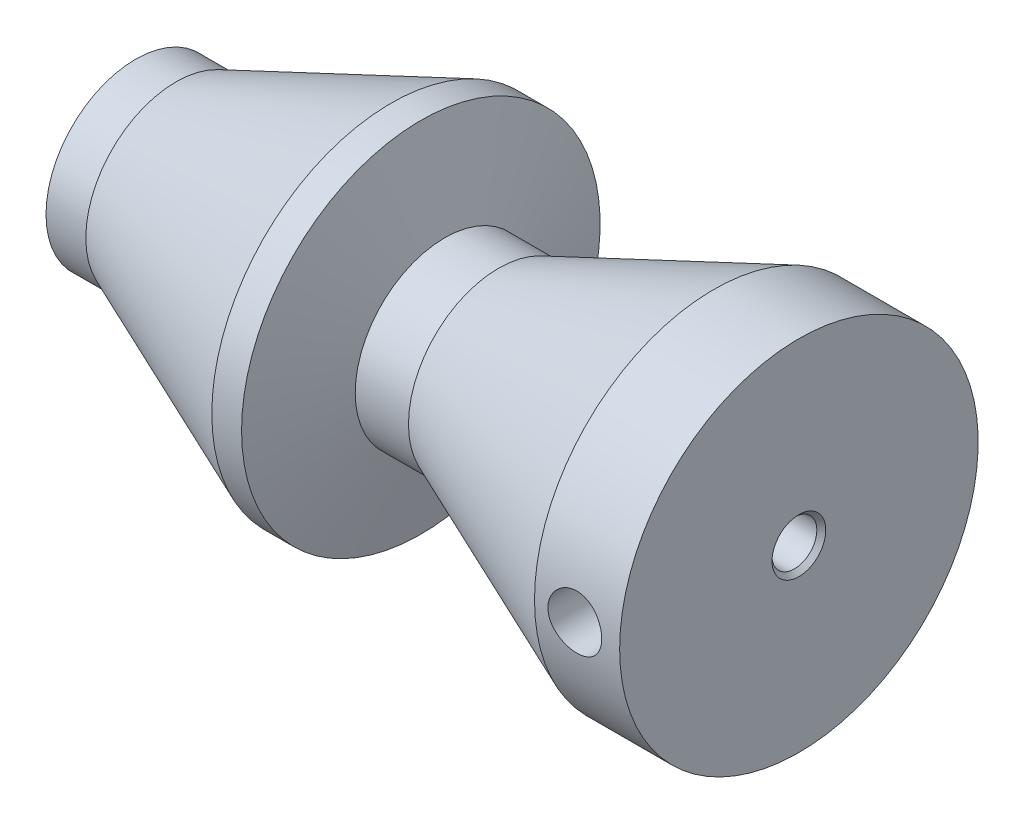
SolidWorks part; units mm, degrees
ref_plane "前视基准面" through (0, 0, 0) normal (0, 0, 1) x (1, 0, 0)
ref_plane "上视基准面" through (0, 0, 0) normal (0, 1, 0) x (1, 0, 0)
ref_plane "右视基准面" through (0, 0, 0) normal (1, 0, 0) x (0, 0, -1)
sketch "草图1" plane through (0, 0, 0) normal (0, 0, 1) x (1, 0, 0)
  line L0 (0, 0) -> (236.8731, 0) construction
  line L1 (4.5, 10) -> (0, 10)
  line L2 (4.5, 10.0589) -> (28.5, 20)
  line L3 (28.5, 20) -> (31.8205, 20)
  line L4 (31.8205, 20) -> (34.5, 10)
  line L5 (34.5, 10) -> (40.5, 10)
  line L6 (40.5, 10.0589) -> (64.5, 20)
  line L7 (64.5, 20) -> (74, 20)
  line L8 (74, 20) -> (74, 0)
  line L9 (40.5, 10.0589) -> (40.5, 10)
  line L10 (0, 10) -> (0, 0)
  line L11 (4.5, 10.0589) -> (4.5, 10)
  line L12 (0, 0) -> (74, 0)
  dimension "D1" = 4.5
  dimension "D2" = 22.5
  dimension "D3" = 74
  dimension "D4" = 9.5
  dimension "D5" = 20
  dimension "D6" = 36
  dimension "D7" = 22.5
  dimension "D8" = 10
  dimension "D9" = 36
  dimension "D10" = 6
  dimension "D11" = 105
revolve "旋转1" add sketch "草图1" angle 360 about L0
hole_wizard "M6 螺纹孔1" positions "草图3" profile "草图2" tap size "M6" standard "GB"
sketch "草图3" plane through (74, 0, 0) normal (1, 0, 0) x (0, 0, -1)
  point P0 (0, 0)
sketch "草图2" plane through (74, 0, 0) normal (0, 1, 0) x (0, 0, -1)
  line L0 (0, 0) -> (0, 18.5022)
  line L1 (0, 18.5022) -> (2.5, 17)
  line L2 (2.5, 17) -> (2.5, 0)
  line L5 (2.5, 0) -> (0, 0)
  line L10 (0, 18.5022) -> (-2.5, 17) construction
  line L11 (0, -6.35) -> (0, 107.95) construction
  dimension "螺纹孔钻头直径" = 5
  dimension "螺纹孔钻头深度" = 17
  dimension "导头角度" = 118
cosmetic thread "孔螺蚊线1" parameters "D1"=12, "D2"=6
chamfer "倒角1" distance 0.5 angle 45 1 edges at (74, 0, -2.5)
hole_wizard "Ø6.0 (6) 直径孔1" positions "3D草图1" profile "草图4" hole size "Ø6.0" standard "GB"
sketch3d "3D草图1"
  point P0 (69, 0, 20)
  dimension "D1" = 5
sketch "草图4" plane through (69, 0, 20) normal (1, 0, 0) x (0, -1, 0)
  line L0 (0, 0) -> (0, 11.8026)
  line L1 (0, 11.8026) -> (3, 10)
  line L2 (3, 10) -> (3, 0)
  line L5 (3, 0) -> (0, 0)
  line L10 (0, 11.8026) -> (-3, 10) construction
  line L11 (0, -6.35) -> (0, 107.95) construction
  dimension "孔直径" = 6
  dimension "孔深度" = 10
  dimension "导头角度" = 118
